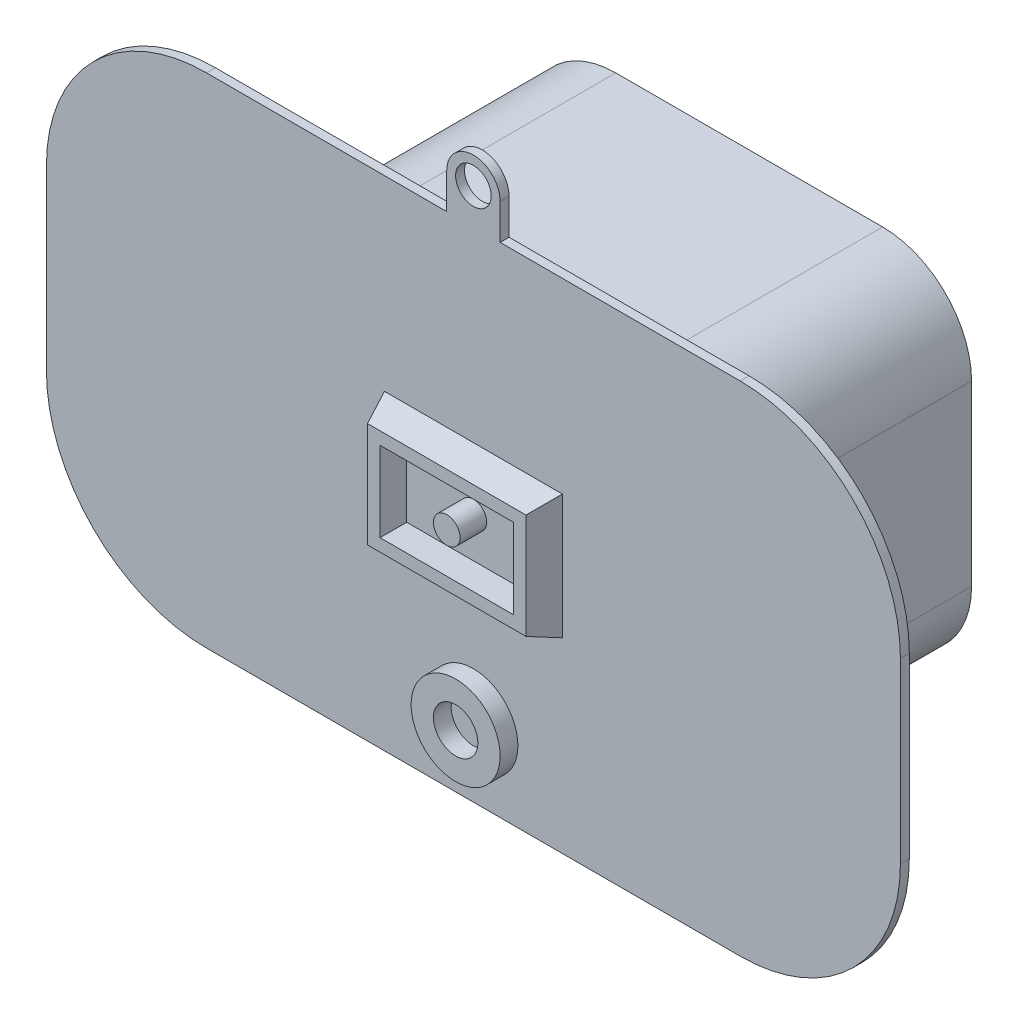
from build123d import *

# Parameters (mm, degrees)
SKETCH1_R           = 2
BOSS_EXTRUDE1_DEPTH = 1
SKETCH2_W           = 20
SKETCH2_H           = 14
BOSS_EXTRUDE2_DEPTH = 3
BOSS_EXTRUDE2_TAPER = 20
SKETCH3_W           = 15
SKETCH3_H           = 9
SKETCH3_R           = 1.5
CUT_EXTRUDE1_DEPTH  = 3
SKETCH4_W           = 50
SKETCH4_H           = 40
SKETCH4_W_2         = 46
SKETCH4_H_2         = 36
BOSS_EXTRUDE3_DEPTH = 30
SKETCH5_R           = 5
SKETCH5_R_2         = 2.5
BOSS_EXTRUDE4_DEPTH = 2
FILLET1_R           = 8
FILLET2_R           = 10


with BuildPart() as part:
    # Sketch1 → Boss-Extrude1 (new body)
    with BuildSketch(Plane.XY):
        with BuildLine():
            Line((-3, 28), (-3, 32))
            ThreePointArc((-3, 32), (0, 35), (3, 32))
            Line((3, 32), (3, 28))
            Line((3, 28), (30, 28))
            ThreePointArc((30, 28), (42.727922061, 22.727922061), (48, 10))
            Line((48, 10), (48, -10))
            ThreePointArc((48, -10), (42.727922061, -22.727922061), (30, -28))
            Line((30, -28), (-30, -28))
            ThreePointArc((-30, -28), (-42.727922061, -22.727922061), (-48, -10))
            Line((-48, -10), (-48, 10))
            ThreePointArc((-48, 10), (-42.727922061, 22.727922061), (-30, 28))
            Line((-30, 28), (-3, 28))
        make_face()
        with Locations((0, 32)):
            Circle(SKETCH1_R, mode=Mode.SUBTRACT)
    extrude(amount=BOSS_EXTRUDE1_DEPTH)

    # Sketch2 → Boss-Extrude2 (add)
    with BuildSketch(Plane.XY.offset(1)):
        Rectangle(SKETCH2_W, SKETCH2_H)
    extrude(amount=BOSS_EXTRUDE2_DEPTH, taper=BOSS_EXTRUDE2_TAPER)

    # Sketch3 → Cut-Extrude1 (cut)
    with BuildSketch(Plane.XY.offset(4)):
        Rectangle(SKETCH3_W, SKETCH3_H)
        Circle(SKETCH3_R, mode=Mode.SUBTRACT)
    extrude(amount=-CUT_EXTRUDE1_DEPTH, mode=Mode.SUBTRACT)

    # Sketch4 → Boss-Extrude3 (add)
    with BuildSketch(Plane(origin=(0, 0, 0), x_dir=(-1, 0, 0), z_dir=(0, 0, -1))):
        Rectangle(SKETCH4_W, SKETCH4_H)
        Rectangle(SKETCH4_W_2, SKETCH4_H_2, mode=Mode.SUBTRACT)
    extrude(amount=BOSS_EXTRUDE3_DEPTH)

    # Sketch5 → Boss-Extrude4 (add)
    with BuildSketch(Plane.XY.offset(1)):
        with Locations((0, -20)):
            Circle(SKETCH5_R)
        with Locations((0, -20)):
            Circle(SKETCH5_R_2, mode=Mode.SUBTRACT)
    extrude(amount=BOSS_EXTRUDE4_DEPTH)

    # Fillet1
    fillet1_edges = [part.edges().sort_by_distance(p)[0] for p in [
        (-23, 18, -15),
        (23, 18, -15),
        (23, -18, -15),
        (-23, -18, -15),
    ]]
    fillet(fillet1_edges, radius=FILLET1_R)

    # Fillet2
    fillet2_edges = [part.edges().sort_by_distance(p)[0] for p in [
        (-25, -20, -15),
        (-25, 20, -15),
        (25, 20, -15),
        (25, -20, -15),
    ]]
    fillet(fillet2_edges, radius=FILLET2_R)


solid = part.part
